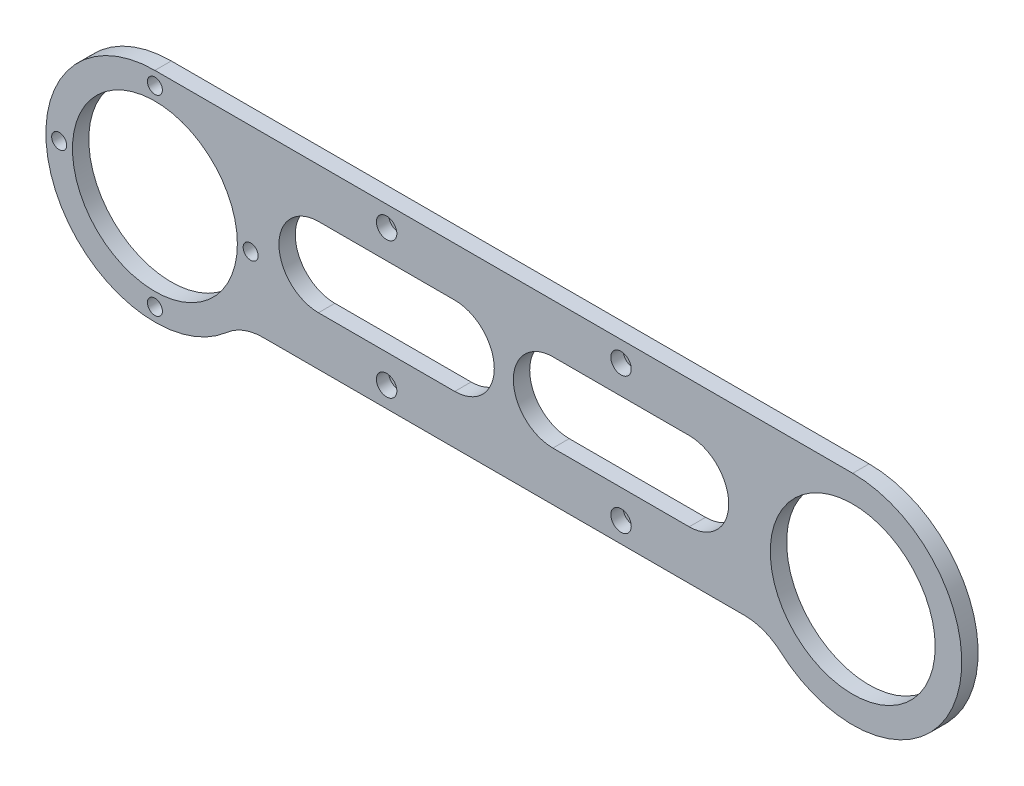
from build123d import *

# Parameters (mm, degrees)
SKETCH_1_R                   = 60.5
EXTRUDE_2_DEPTH              = 12
CUT_EXTRUDE_START            = 8
SKETCH_3_R                   = 60.5
CUT_EXTRUDE_2_DEPTH          = 339.956913315
SKETCH_5_R                   = 18
CUT_EXTRUDE_3_DEPTH          = 347.956913315
HOLE_WIZARD_M8_1_D           = 9
HOLE_WIZARD_M8_1_CBORE_D     = 15
HOLE_WIZARD_M8_1_CBORE_DEPTH = 9
SKETCH_9_R                   = 5.5
CUT_EXTRUDE_4_DEPTH          = 347.956913315
SKETCH_10_R                  = 60.5
CUT_EXTRUDE_5_DEPTH          = 347.841606064


with BuildPart() as part:
    # 草图1 → 凸台-拉伸2 (new body)
    with BuildSketch(Plane.XY):
        with BuildLine():
            Line((-256, 85.668545552), (256, 85.668545552))
            ThreePointArc((256, 85.668545552), (330.833147735, -22.615725695), (203.084973779, -54.331454448))
            ThreePointArc((203.084973779, -54.331454448), (190.769596292, -46.91488058), (176.627460668, -44.331454448))
            Line((176.627460668, -44.331454448), (-176.627460668, -44.331454448))
            ThreePointArc((-176.627460668, -44.331454448), (-190.769596292, -46.91488058), (-203.084973779, -54.331454448))
            ThreePointArc((-203.084973779, -54.331454448), (-330.833147735, -22.615725695), (-256, 85.668545552))
        make_face()
        with Locations((-256, 5.668545552)):
            Circle(SKETCH_1_R, mode=Mode.SUBTRACT)
        with BuildLine():
            Line((36, 49.668545552), (136, 49.668545552))
            ThreePointArc((136, 49.668545552), (165, 20.668545552), (136, -8.331454448))
            Line((136, -8.331454448), (36, -8.331454448))
            ThreePointArc((36, -8.331454448), (7, 20.668545552), (36, 49.668545552))
        make_face(mode=Mode.SUBTRACT)
        with BuildLine():
            Line((-136, 49.668545552), (-36, 49.668545552))
            ThreePointArc((-36, 49.668545552), (-7, 20.668545552), (-36, -8.331454448))
            Line((-36, -8.331454448), (-136, -8.331454448))
            ThreePointArc((-136, -8.331454448), (-165, 20.668545552), (-136, 49.668545552))
        make_face(mode=Mode.SUBTRACT)
    extrude(amount=EXTRUDE_2_DEPTH)

    # 草图3 → 切除-拉伸2 (cut, through all)
    with BuildSketch(Plane.XY.offset(CUT_EXTRUDE_START)):
        with Locations((256, 5.668545552)):
            Circle(SKETCH_3_R)
    extrude(amount=CUT_EXTRUDE_2_DEPTH, mode=Mode.SUBTRACT)

    # 草图5 → 切除-拉伸3 (cut, through all)
    with BuildSketch(Plane.XY):
        with Locations((256, 5.668545552)):
            Circle(SKETCH_5_R)
    extrude(amount=CUT_EXTRUDE_3_DEPTH, mode=Mode.SUBTRACT)

    # M8 六角圆柱头螺钉的柱形沉头孔1 (through all)
    with Locations(Plane.XY.offset(12)):
        with Locations((-86, 70.668545552), (-86, -29.331454448), (86, 70.668545552), (86, -29.331454448)):
            CounterBoreHole(HOLE_WIZARD_M8_1_D / 2, HOLE_WIZARD_M8_1_CBORE_D / 2, HOLE_WIZARD_M8_1_CBORE_DEPTH)

    # 草图9 → 切除-拉伸4 (cut, through all)
    with BuildSketch(Plane(origin=(0, 0, 0), x_dir=(-1, 0, 0), z_dir=(0, 0, -1))):
        with Locations((256, 75.918545552)):
            Circle(SKETCH_9_R)
        with Locations((326.25, 5.668545552)):
            Circle(SKETCH_9_R)
        with Locations((256, -64.581454448)):
            Circle(SKETCH_9_R)
        with Locations((185.75, 5.668545552)):
            Circle(SKETCH_9_R)
    extrude(amount=-CUT_EXTRUDE_4_DEPTH, mode=Mode.SUBTRACT)

    # 草图10 → 切除-拉伸5 (cut, through all)
    with BuildSketch(Plane.XY.offset(8)):
        with Locations((256, 5.668545552)):
            Circle(SKETCH_10_R)
    extrude(amount=-CUT_EXTRUDE_5_DEPTH, mode=Mode.SUBTRACT)


solid = part.part
